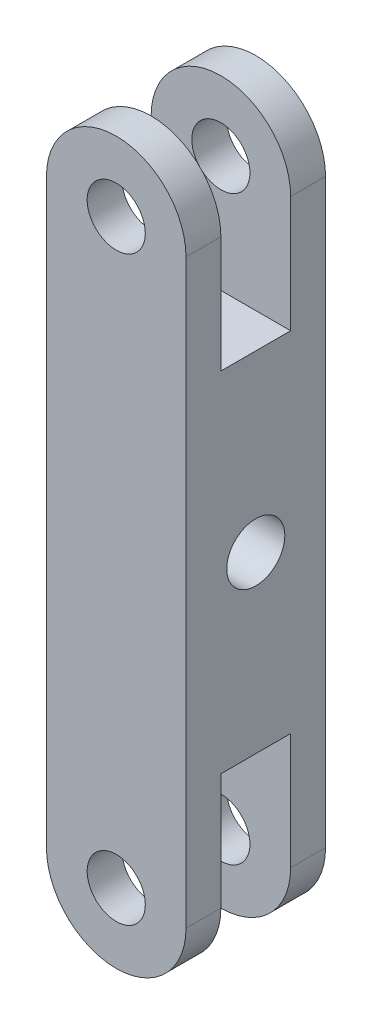
from build123d import *

# Parameters (mm, degrees)
BOSS_EXTRUDE1_DEPTH = 12
SKETCH2_W           = 6
SKETCH2_H           = 32
CUT_EXTRUDE1_DEPTH  = 59.514955353
SKETCH3_R           = 2.5
CUT_EXTRUDE2_DEPTH  = 58.584720196
M6_TAPPED_HOLE1_D   = 5


with BuildPart() as part:
    # Sketch1 → Boss-Extrude1 (new body)
    with BuildSketch(Plane.XY):
        with BuildLine():
            Line((-6, 0), (-6, 50))
            ThreePointArc((-6, 50), (0, 56), (6, 50))
            Line((6, 50), (6, 0))
            ThreePointArc((6, 0), (0, -6), (-6, 0))
        make_face()
    extrude(amount=BOSS_EXTRUDE1_DEPTH)

    # Sketch2 → Cut-Extrude1 (cut, through all)
    with BuildSketch(Plane.ZY.offset(6)):
        with Locations((6, 56)):
            Rectangle(SKETCH2_W, SKETCH2_H)
        with Locations((6, -6)):
            Rectangle(SKETCH2_W, SKETCH2_H)
    extrude(amount=-CUT_EXTRUDE1_DEPTH, mode=Mode.SUBTRACT)

    # Sketch3 → Cut-Extrude2 (cut, through all)
    with BuildSketch(Plane.XY.offset(12)):
        with Locations((0, 50)):
            Circle(SKETCH3_R)
        Circle(SKETCH3_R)
    extrude(amount=-CUT_EXTRUDE2_DEPTH, mode=Mode.SUBTRACT)

    # M6 Tapped Hole1 (through all)
    with Locations(Plane(origin=(6, 25, 6), x_dir=(0, 0, 1), z_dir=(1, 0, 0))):
        with Locations((0, 0)):
            Hole(M6_TAPPED_HOLE1_D / 2)


solid = part.part
